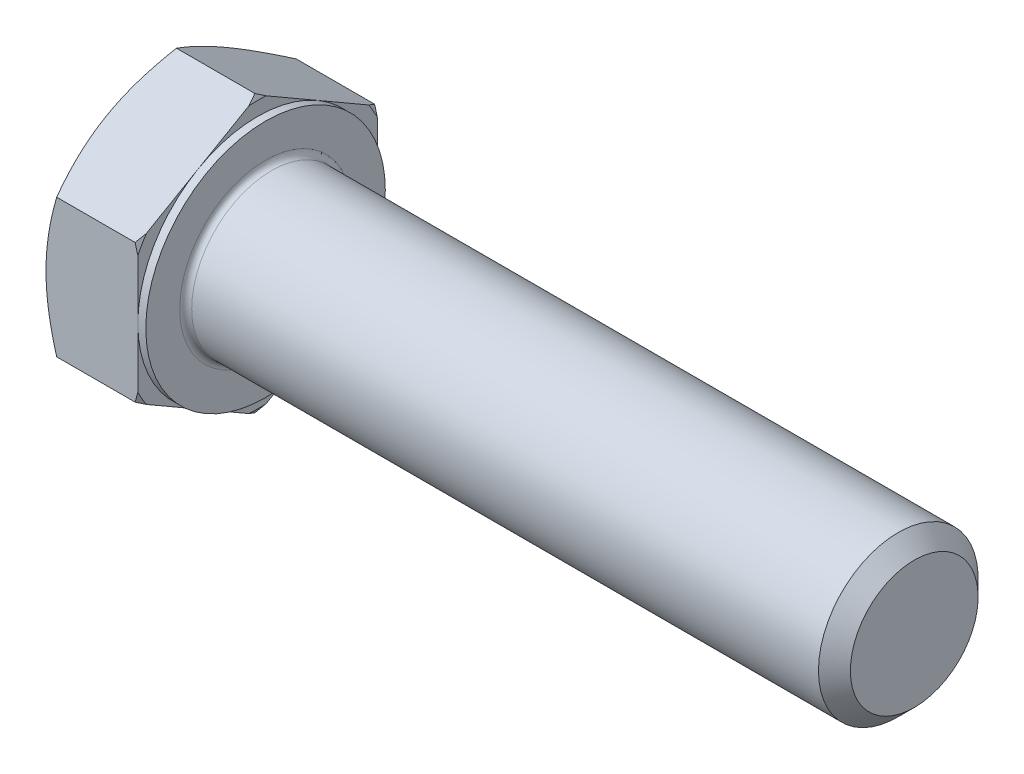
from build123d import *

# Parameters (mm, degrees)
EXTRUDE_365_DEPTH = 10
SKETCH_4_W        = 0.8
SKETCH_4_H        = 11.856406461
CHAMFER_2062_SIZE = 1.6
FILLET_2107_R     = 0.6


with BuildPart() as part:
    # 草图1 → Extrude 365 (new body)
    with BuildSketch(Plane(origin=(0, 0, 0), x_dir=(0, 0, -1), z_dir=(1, 0, 0))):
        Polygon((12, 6.92820323), (12, -6.92820323), (0, -13.856406461), (-12, -6.92820323), (-12, 6.92820323), (0, 13.856406461), align=None)
    extrude(amount=EXTRUDE_365_DEPTH)

    # 草图2 → 凸台-旋转1 (revolve)
    with BuildSketch(Plane.XY, mode=Mode.PRIVATE) as revolve_1_sk:
        Polygon((0, 0), (75, 0), (75, 6.268), (75, 8), (7.791693541, 8), (0, 8), align=None)
    revolve(revolve_1_sk.sketch.rotate(Axis((0, 0, 0), (1, 0, 0)), 90), axis=Axis((0, 0, 0), (1, 0, 0)))

    # 草图3 → 切除-旋转1 (revolve, cut)
    with BuildSketch(Plane.XY):
        Polygon((0, 12), (3.958548116, 18.856406461), (3.958548116, 23.856406461), (-10, 23.856406461), (-10, 12), align=None)
    revolve(axis=Axis((0, 0, 0), (1, 0, 0)), mode=Mode.SUBTRACT)

    # 草图5 → 切除-旋转2 (revolve, cut)
    with BuildSketch(Plane.XY):
        Polygon((10, 12), (6.041451884, 18.856406461), (6.041451884, 23.856406461), (16.041451884, 23.856406461), (16.041451884, 12), align=None)
    revolve(axis=Axis((0, 0, 0), (1, 0, 0)), mode=Mode.SUBTRACT)

    # 草图4 → 切除-旋转3 (revolve, cut)
    with BuildSketch(Plane.XY, mode=Mode.PRIVATE) as cut_revolve_3_sk:
        with Locations((9.6, 17.928203231)):
            Rectangle(SKETCH_4_W, SKETCH_4_H)
    revolve(cut_revolve_3_sk.sketch.rotate(Axis((0, 0, 0), (1, 0, 0)), 270), axis=Axis((0, 0, 0), (1, 0, 0)), mode=Mode.SUBTRACT)

    # Chamfer 2062
    chamfer_2062_edges = [part.edges().sort_by_distance(p)[0] for p in [
        (75, 0, -8),
    ]]
    chamfer(chamfer_2062_edges, length=CHAMFER_2062_SIZE)

    # Fillet 2107
    fillet_2107_edges = [part.edges().sort_by_distance(p)[0] for p in [
        (10, 0, -8),
    ]]
    fillet(fillet_2107_edges, radius=FILLET_2107_R)


solid = part.part
